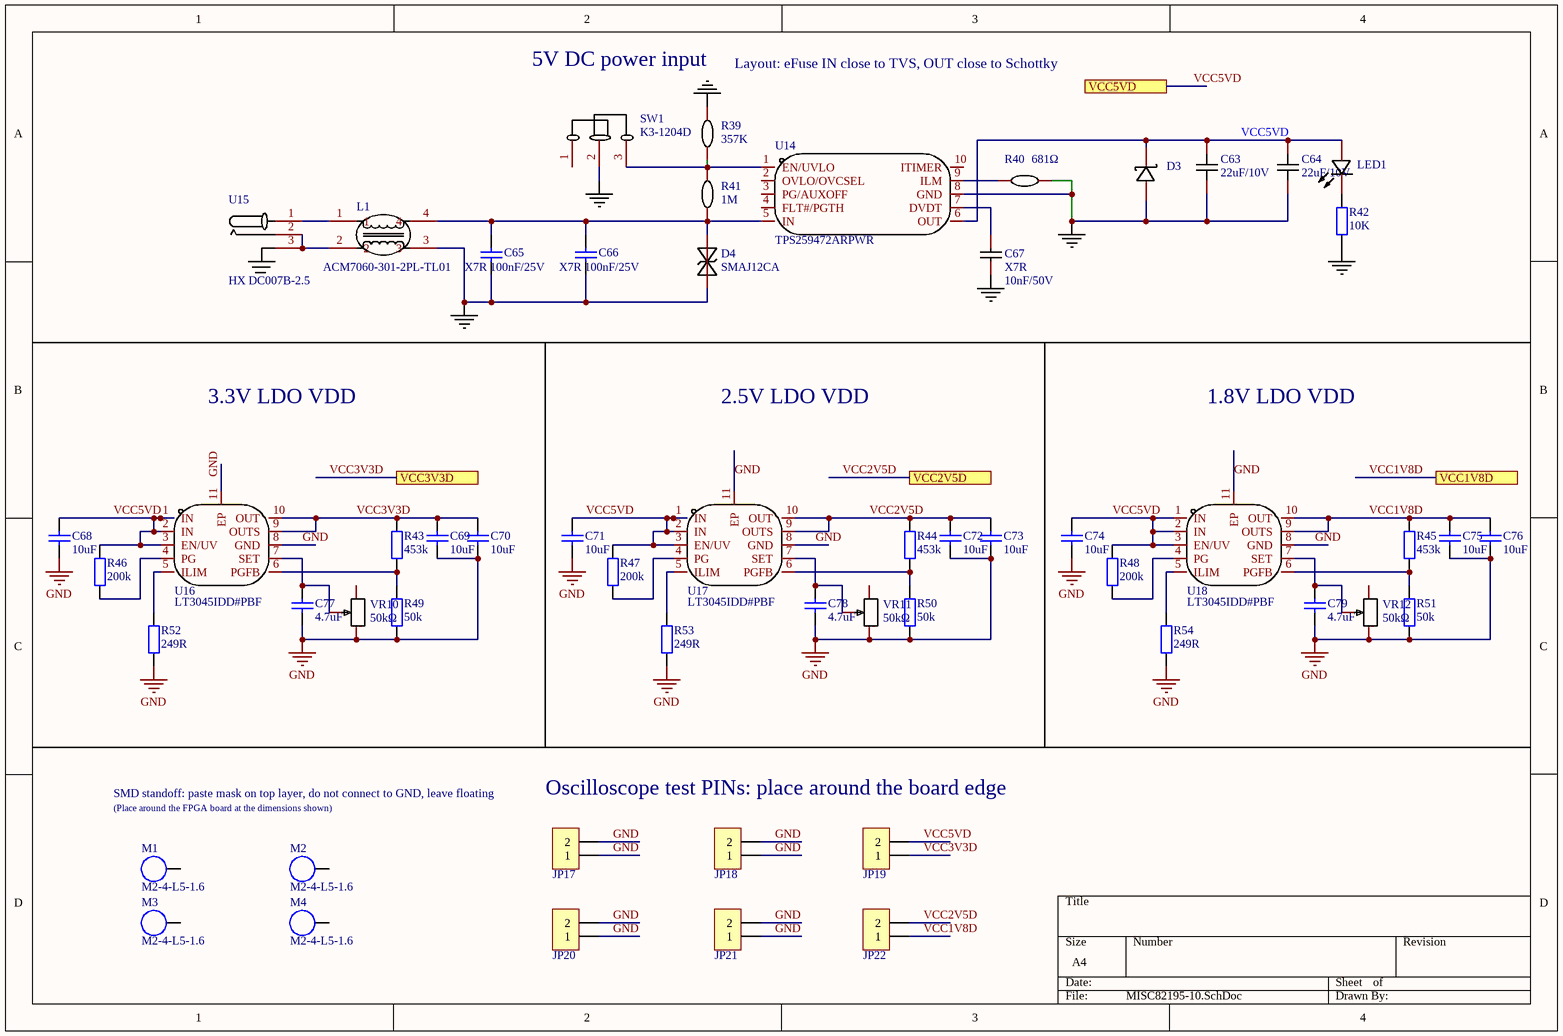
[diagram p0: MISC82195-10.SchDoc]
# Altium project MISC82195-8.PrjPcb (part 2 of 2)

## Sheet MISC82195-10.SchDoc
size A4; SheetNumber: 3; SheetTotal: 3

### Parts
C63  22uF/10V  [C0603]
C64  22uF/10V  [C0603]
C65  X7R 100nF/25V  [C0603]
C66  X7R 100nF/25V  [C0603]
C67  X7R  Name: 10nF/50V  [C0603]
C68  10uF  [C0603]
C69  10uF  [C0603]
C70  10uF  [C0603]
C71  10uF  [C0603]
C72  10uF  [C0603]
C73  10uF  [C0603]
C74  10uF  [C0603]
C75  10uF  [C0603]
C76  10uF  [C0603]
C77  4.7uF  [C0603]
C78  4.7uF  [C0603]
C79  4.7uF  [C0603]
D3  VS-10BQ015HM3/5BT  [SMB_L4.6-W3.6-LS5.3-RD]  (value not drawn)
D4  SMAJ12CA  [SMA_L4.2-W2.7-LS5.0-BI]
JP17  HDR-1X2  [HDR2.54-LI-2P]  (value not drawn)
JP18  HDR-1X2  [HDR2.54-LI-2P]  (value not drawn)
JP19  HDR-1X2  [HDR2.54-LI-2P]  (value not drawn)
JP20  HDR-1X2  [HDR2.54-LI-2P]  (value not drawn)
JP21  HDR-1X2  [HDR2.54-LI-2P]  (value not drawn)
JP22  HDR-1X2  [HDR2.54-LI-2P]  (value not drawn)
L1  ACM7060-301-2PL-TL01  [FILTER-SMD_4P-L7.0-W6.0-TL_SMCM7060]
LED1  NCD0805G1  [LED0805-R-RD]  (value not drawn)
M1  M2-4-L5-1.6  [M2.9]
M2  M2-4-L5-1.6  [M2.9]
M3  M2-4-L5-1.6  [M2.9]
M4  M2-4-L5-1.6  [M2.9]
R39  357K  [R0603]
R40  681Ω  [R0603]
R41  1M  [R0603]
R42  10K  [R0603]
R43  453k  [R0603]
R44  453k  [R0603]
R45  453k  [R0603]
R46  200k  [R0603]
R47  200k  [R0603]
R48  200k  [R0603]
R49  50k  [R0603]
R50  50k  [R0603]
R51  50k  [R0603]
R52  249R  [R0603]
R53  249R  [R0603]
R54  249R  [R0603]
SW1  K3-1204D  [SW-TH_K3-1204D]
U14  TPS259472ARPWR  [VQFN-10_L2.0-W2.0-P0.45-TL]
U15  HX DC007B-2.5  [DC-IN-TH_HX-DC007B-2.5]
U16  LT3045IDD#PBF  [DFN-10_L3.0-W3.0-P0.50-BL-EP-3]
U17  LT3045IDD#PBF  [DFN-10_L3.0-W3.0-P0.50-BL-EP-3]
U18  LT3045IDD#PBF  [DFN-10_L3.0-W3.0-P0.50-BL-EP-3]
VR10  50kΩ  [RES-ADJ-SMD_3224W]
VR11  50kΩ  [RES-ADJ-SMD_3224W]
VR12  50kΩ  [RES-ADJ-SMD_3224W]

### Ports
VCC1V8D, VCC2V5D, VCC3V3D, VCC5VD

### Nets
GND: C63.1 C64.1 C65.1 C66.1 C67.1 C68.1 C69.1 C70.1 C71.1 C72.1 C73.1 C74.1 C75.1 C76.1 C77.1 C78.1 C79.1 D3.2(A) D4.1 JP17.1 JP17.2 JP18.1 JP18.2 JP20.1 JP20.2 JP21.1 JP21.2 L1.3 R39.2 R40.2 R42.1 R49.1 R50.1 R51.1 R52.1 R53.1 R54.1 SW1.2 U14.8(GND) U16.8(GND) U16.11(EP) U17.8(GND) U17.11(EP) U18.8(GND) U18.11(EP) VR10.3 VR11.3 VR12.3
VCC1V8D: C75.2 C76.2 JP22.1 R45.2 U18.9(OUTS) U18.10(OUT) ; port VCC1V8D
VCC3V3D: C69.2 C70.2 JP19.1 R43.2 U16.9(OUTS) U16.10(OUT) ; port VCC3V3D
VCC5VD: C63.2 C64.2 C68.2 C71.2 C74.2 D3.1(C) JP19.2 LED1.1(A) R46.2 R47.2 R48.2 U14.6(OUT) U16.1(IN) U16.2(IN) U16.3(EN/UV) U17.1(IN) U17.2(IN) U17.3(EN/UV) U18.1(IN) U18.2(IN) U18.3(EN/UV) ; port VCC5VD
VCC2V5D: C72.2 C73.2 JP22.2 R44.2 U17.9(OUTS) U17.10(OUT) ; port VCC2V5D
NetC65_2: C65.2 C66.2 D4.2 L1.4 R41.1 U14.5(IN)
NetC67_2: C67.2 U14.7(DVDT)
NetC77_2: C77.2 U16.7(SET) VR10.2
NetC78_2: C78.2 U17.7(SET) VR11.2
NetC79_2: C79.2 U18.7(SET) VR12.2
NetL1_1: L1.1 U15.1
NetL1_2: L1.2 U15.2 U15.3
NetLED1_2: LED1.2(K) R42.2
NetR39_1: R39.1 R41.2 SW1.3 U14.1(EN/UVLO)
NetR40_1: R40.1 U14.9(ILM)
NetR43_1: R43.1 R49.2 U16.6(PGFB)
NetR44_1: R44.1 R50.2 U17.6(PGFB)
NetR45_1: R45.1 R51.2 U18.6(PGFB)
NetR46_1: R46.1 U16.4(PG)
NetR47_1: R47.1 U17.4(PG)
NetR48_1: R48.1 U18.4(PG)
NetR52_2: R52.2 U16.5(ILIM)
NetR53_2: R53.2 U17.5(ILIM)
NetR54_2: R54.2 U18.5(ILIM)

Not connected (* = marked no-connect by the designer): M1 1; M2 1; M3 1; M4 1; SW1 1; U14 2(OVLO/OVCSEL) 3(PG/AUXOFF) 4(FLT#/PGTH) 10(ITIMER); VR10 1; VR11 1; VR12 1

### Notes on the sheet
- 5V DC power input
- Layout: eFuse IN close to TVS, OUT close to Schottky
- 3.3V LDO VDD
- 2.5V LDO VDD
- 1.8V LDO VDD
- (near JP17) SMD standoff: paste mask on top layer, do not connect to GND, leave floating
- (Place around the FPGA board at the dimensions shown)
- Oscilloscope test PINs: place around the board edge

### Library data of the parts
C63 C64 = CL21A226MAQNNNE: Manufacturer: SAMSUNG(三星); Add into BOM: yes; Tolerance: ±20%; Voltage Rated: 25V; Temperature Coefficient: X5R; Name: 22uF/10V; Symbol: CL21A226MAQNNNE; Device: CL21A226MAQNNNE; Supplier: LCSC; Manufacturer Part: CL21A226MAQNNNE; Value: 22uF/10V; Supplier Part: C45783; JLCPCB Part Class: Basic library; LCSC Part Name: 22uF ±20% 25V; Supplier Footprint: 0805; Datasheet: https://atta.szlcsc.com/upload/public/pdf/source/20160218/1457707763339.pdf; Convert to PCB: yes
C65 C66 C68-C79 = C: SMD capacitor; BOM名称: Non-polar SMD capacitor
C67 = CC0603KRX7R9BB103: Manufacturer: YAGEO(国巨); Value: 10nF/50V; Add into BOM: yes; Tolerance: ±10%; Voltage Rated: 50V; Symbol: CC0603KRX7R9BB103; Device: CC0603KRX7R9BB103; Supplier: LCSC; Manufacturer Part: CC0603KRX7R9BB103; Supplier Part: C100042; JLCPCB Part Class: Extended library; LCSC Part Name: 10nF ±10% 50V; Supplier Footprint: 0603; Datasheet: https://atta.szlcsc.com/upload/public/pdf/source/20181008/C309510_22F155564471FAF6A489F7D68F34234E.pdf; Convert to PCB: yes; Temperature Coefficient: X7R
D3 = VS-10BQ015HM3/5BT: Manufacturer: VISHAY(威世); Add into BOM: yes; Forward Voltage (Vf@If): 210mV@1A; Reverse Voltage (Vr): 15V; Average Rectified Current (Io): 1A; Reverse Leakage Current (Ir): 500uA@15V; Name: VS-10BQ015HM3/5BT; Symbol: VS-10BQ015HM3/5BT; Device: VS-10BQ015HM3/5BT; Supplier: LCSC; Supplier Part: C413465; Manufacturer Part: VS-10BQ015HM3/5BT; JLCPCB Part Class: Extended library; LCSC Part Name: 电压:15V 电流:1A; Supplier Footprint: DO-214AA(SMB); Datasheet: https://atta.szlcsc.com/upload/public/pdf/source/20190819/C413465_3D2B1A8C7366D4425AB887DF85498F89.pdf; Convert to PCB: yes
D4 = SMAJ12CA_C908818: Manufacturer: GOODWORK(固得沃克); Add into BOM: yes; Reverse Stand-Off Voltage (Vrwm): 12V; Maximum Clamping Voltage: 19.9V; Peak Pulse Current (Ipp)@10/1000us: 20.1A; Breakdown Voltage: 13.3V; Reverse Leakage Current (Ir): 5uA; Type: TVS; Name: SMAJ12CA; Symbol: SMAJ12CA_C908818; Device: SMAJ12CA_C908818; Supplier: LCSC; Supplier Part: C908818; Manufacturer Part: SMAJ12CA; JLCPCB Part Class: Extended library; LCSC Part Name: 双向TVS 12V截止 20.1A峰值脉冲; Supplier Footprint: SMA(DO-214AC); Datasheet: https://atta.szlcsc.com/upload/public/pdf/source/20201231/C908757_5436EAF671B686EFC2F0DD2098F0ED89.pdf; Convert to PCB: yes
JP17-JP22 = Header 2: 2P connector; BOM名称: 2P connector
L1 = ACM7060-301-2PL-TL01: Manufacturer: TDK; Value: 300Ω; Add into BOM: yes; Number of Lines: 2; Current Rating: 5A; Voltage Rating - DC: 80V; Impedance @ Frequency: 300Ω@100MHz; DC Resistance (DCR): 10mΩ; Name: ACM7060-301-2PL-TL01; Symbol: ACM7060-301-2PL-TL01; Device: ACM7060-301-2PL-TL01; Supplier: LCSC; Manufacturer Part: ACM7060-301-2PL-TL01; Supplier Part: C76580; JLCPCB Part Class: Extended library; LCSC Part Name: 两路 贴片共模滤波器 阻抗300Ω@100MHz; Supplier Footprint: SMD,7x6mm; Datasheet: https://atta.szlcsc.com/upload/public/pdf/source/20160918/1474166841345.pdf; Convert to PCB: yes; Operating Temperature: -40℃~+85℃
LED1 = NCD0805G1: Manufacturer: 国星光电; Symbol: FC-2012UGK-520D5; Add into BOM: yes; Emitted Color: Emerald green; Forward Voltage (VF): 2.5V~3.6V; Power Dissipation: 72mW; Forward Current: 5mA; Dominant Wavelength: 525nm~537.5nm; Lens Color: Colorless transparent lens; Luminous Intensity: 180mcd~400mcd; Viewing Angle: 130°; Name: NCD0805G1; Device: NCD0805G1; Supplier: LCSC; Manufacturer Part: NCD0805G1; Supplier Part: C84260; JLCPCB Part Class: Extended library; LCSC Part Name: NCD0805G1; Supplier Footprint: 0805; Datasheet: https://atta.szlcsc.com/upload/public/pdf/source/20200820/C84260_AFC7BF57C6FBA034D182BB8D10A67EFE.pdf; Convert to PCB: yes; Operating Temperature: -30℃~+85℃
M1-M4 = M2: SMD standoff
R39 R41 = Res_0603: Symbol: Resistor; Convert to PCB: yes; Device: Res_0603; Add into BOM: yes; Supplier Footprint: 0603
  R39: Name: 357K; Value: 357K
  R41: Name: 1M; Value: 1M
R40 = CR0805F681RP05Z: Manufacturer: EVER OHMS(天二科技); Add into BOM: yes; Tolerance: ±1%; Power(Watts): 125mW; Overload Voltage (Max): 150V; Temperature Coefficient: ±100ppm/℃; Name: 681Ω; Symbol: CR0805F681RP05; Device: CR0805F681RP05Z; LCSC Part Name: 厚膜电阻 681Ω ±1% 125mW; Supplier Part: C245369; Manufacturer Part: CR0805F681RP05Z; Supplier Footprint: 0805; JLCPCB Part Class: Extended library; Datasheet: https://atta.szlcsc.com/upload/public/pdf/source/20190724/C171430_9E147A274D2811BD276FBB11C8CE6534.pdf; Supplier: LCSC; Convert to PCB: yes; Type: Thick-film resistor; Value: 681Ω; Operating Temperature Range: -55℃~+155℃
R42-R54 = R: SMD resistor; BOM名称: SMD resistor
SW1 = K3-1204D: Manufacturer: 韩国韩荣; Add into BOM: yes; Circuit: Single-pole double-throw; Pin Style: PCB pin; Switch Length: 10mm; Switch Width: 2.5mm; Switch Height: 6mm; Actuator Color: Red; Current Rating (AC): 5A; Voltage Rating (AC): 120V; Mechanical Life: 5万次; Name: K3-1204D; Symbol: K3-1204D; Device: K3-1204D; LCSC Part Name: 直插双档 滑动开关; Supplier Part: C145861; Manufacturer Part: K3-1204D; Supplier Footprint: 插件; JLCPCB Part Class: Extended library; Datasheet: https://atta.szlcsc.com/upload/public/pdf/source/20210810/A7BCE8A3AE6875067403B729968221B7.pdf; Supplier: LCSC; Convert to PCB: yes; Actuator Style: -; Mounting Style: Through-hole; Voltage Rating (DC): -; Operating Temperature: -25℃~+80℃
U14 = TPS259472ARPWR: Manufacturer: TI(德州仪器); Add into BOM: yes; Voltage Rating: 2.7V~23V; Name: TPS259472ARPWR; Symbol: TPS259472ARPWR; Device: TPS259472ARPWR; LCSC Part Name: TPS259472ARPWR; Supplier Part: C3662789; Manufacturer Part: TPS259472ARPWR; Supplier Footprint: VQFN-10-HR(2x2); JLCPCB Part Class: Extended library; Datasheet: https://www.ti.com/cn/lit/gpn/tps25947; Supplier: LCSC; Convert to PCB: yes; Operating temperature: -40℃~+125℃
U15 = HX DC007B-2.5: Manufacturer: hanxia(韩下); Add into BOM: yes; Connector Type: DC power socket; Inside Contact Diameter: 2.5mm; Outside Contact Diameter: 6.4mm; Current Rating (Max): 7A; Voltage Rating (Max): 20V; Name: HX DC007B-2.5; Symbol: HX DC007B-2.5; Device: HX DC007B-2.5; Supplier: LCSC; Supplier Part: C19189083; Manufacturer Part: HX DC007B-2.5; LCSC Part Name: DC电源插座 内径:2.5mm 外径:6.4mm; Supplier Footprint: 插件; Datasheet: https://atta.szlcsc.com/upload/public/pdf/source/20231103/814B3421283469BAAEFFF9B7A53EC0CB.pdf; Convert to PCB: yes; Mounting Style: Right-angle; Operating Temperature Range: -25℃~+70℃
U16-U18 = LT3045IDD#PBF: Manufacturer: ADI(亚德诺); Add into BOM: yes; Output Type: Adjustable; Maximum Input Voltage: 20V; Output Voltage: 0V~15V; MAX Output Current: 500mA; Dropout Voltage: 450mV@(500mA); standby current: 20uA; Output Polarity: Positive; Number of Outputs: 1; Name: LT3045IDD#PBF; Symbol: LT3045IDD#PBF; Device: LT3045IDD#PBF; LCSC Part Name: LT3045IDD#PBF; Supplier Part: C580013; Manufacturer Part: LT3045IDD#PBF; Supplier Footprint: DFN-10-EP(3x3); JLCPCB Part Class: Extended library; Datasheet: https://atta.szlcsc.com/upload/public/pdf/source/20200416/C514420_E440C492D6C74EAE6AB301243586F696.pdf; Supplier: LCSC; Convert to PCB: yes; Operating Temperature: -40℃~+125℃@(Tj)
VR10-VR12 = 3224W-1-503E: Manufacturer: BOURNS; Resistance: 50K; Add into BOM: yes; Tolerance: ±10%; Power(Watts): 250mW; Temperature Coefficient: ±100ppm/℃; Turns: 12; Name: 50kΩ; Symbol: 3224W-1-503E; Device: 3224W-1-503E; Supplier: LCSC; Manufacturer Part: 3224W-1-503E; Supplier Part: C48484; Value: 50kΩ; JLCPCB Part Class: Extended library; LCSC Part Name: 50kΩ ±10%; Supplier Footprint: SMD; Datasheet: https://atta.szlcsc.com/upload/public/pdf/source/20160830/1472551532733.pdf; Convert to PCB: yes

## Nets that join several sheets
GND: MISC82195-4 (84 pins), MISC82195-2 (129 pins), MISC82195-10 (48 pins)
VCC1V8D: MISC82195-4 (11 pins), MISC82195-2 (C55.2 C56.2 JP14.1), MISC82195-10 (6 pins)
VCC3V3D: MISC82195-4 (12 pins), MISC82195-10 (6 pins)
VCC5VD: MISC82195-4 (9 pins), MISC82195-2 (59 pins), MISC82195-10 (21 pins)
CS_CDAC1: MISC82195-4 (JP5.2 P1.B34), MISC82195-2 (D1.6 D2.6)
CS_DAC1: MISC82195-4 (JP2.7 P2.A26), MISC82195-2 (U11.12)
CS_DAC2: MISC82195-4 (JP2.9 P2.A30), MISC82195-2 (U12.12)
CS_DAC3: MISC82195-4 (JP2.11 P2.A36), MISC82195-2 (U13.12)
PW1: MISC82195-4 (JP2.1 P2.A12), MISC82195-2 (U11.13 U12.13 U13.13)
PW2: MISC82195-4 (JP2.3 P2.A16), MISC82195-2 (U11.14 U12.14 U13.14)
PW3: MISC82195-4 (JP2.5 P2.A20), MISC82195-2 (U11.15 U12.15 U13.15)
PW91: MISC82195-4 (JP5.6 P1.B44), MISC82195-2 (D1.8 D2.8)
PW92: MISC82195-4 (JP5.4 P1.B38), MISC82195-2 (D1.7 D2.7)
PW94: MISC82195-4 (JP3.13 P1.B16), MISC82195-2 (D1.5 D2.5)
VCC2V5D: MISC82195-4 (JP1.4 JP8.4), MISC82195-10 (6 pins)